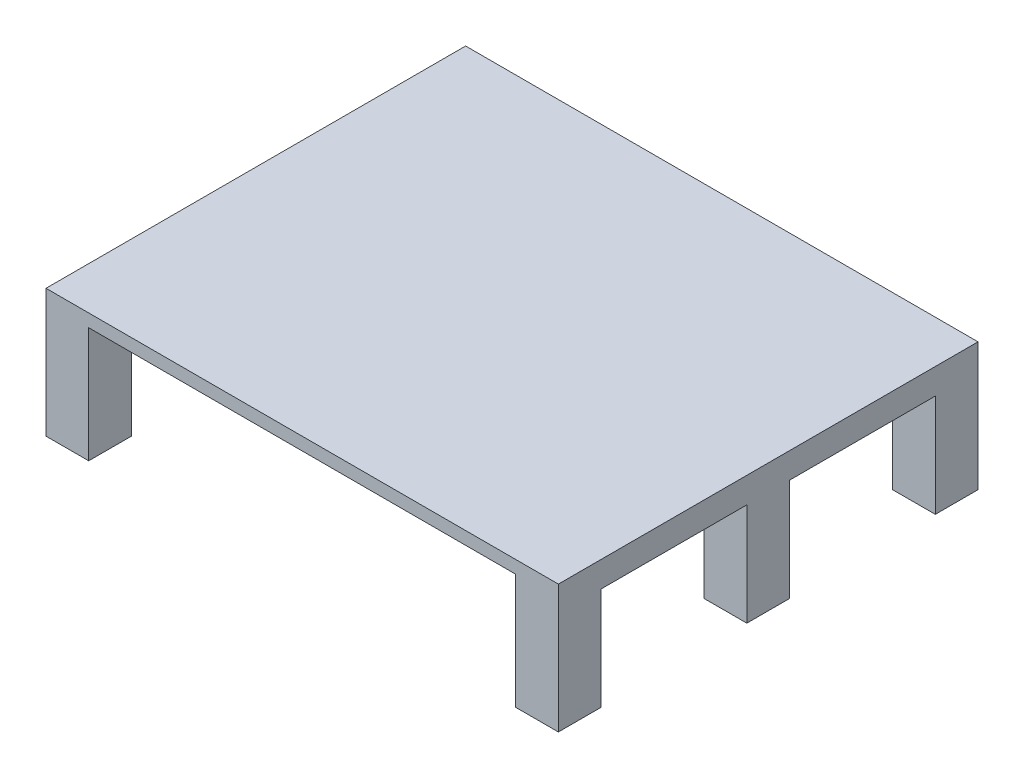
SolidWorks part; units mm, degrees
ref_plane "Front Plane" through (0, 0, 0) normal (0, 0, 1) x (1, 0, 0)
ref_plane "Top Plane" through (0, 0, 0) normal (0, 1, 0) x (1, 0, 0)
ref_plane "Right Plane" through (0, 0, 0) normal (1, 0, 0) x (0, 0, -1)
sketch "Sketch2" plane through (0, 0, 0) normal (0, 0, 1) x (1, 0, 0)
  line L1 (3000, -1500) -> (2500, -1500)
  line L2 (3000, -1500) -> (3000, 0)
  line L3 (3000, 0) -> (-3000, 0)
  line L4 (-3000, -1500) -> (-3000, 0)
  line L5 (0, 0) -> (0, -3054.8137) construction
  line L8 (-2500, -1500) -> (-2500, -150)
  line L9 (-2500, -150) -> (2500, -150)
  line L10 (2500, -1500) -> (2500, -150)
  line L11 (-2500, -1500) -> (-3000, -1500)
  point P0 (0, 0)
  point P6 (0, 0)
  point P11 (2750, -1500)
  dimension "D1" = 1500
  dimension "D2" = 6000
  dimension "D3" = 1350
  dimension "D4" = 5000
extrude "Boss-Extrude1" add sketch "Sketch2" along normal blind 435 and the other way blind 4479
sketch "Sketch3" plane through (3000, 0, 0) normal (1, 0, 0) x (0, 0, -1)
  line L0 (4479, -1500) -> (-435, -1500) construction
  line L1 (65, -1500) -> (1772, -1500)
  line L2 (65, -1500) -> (65, -300)
  line L3 (65, -300) -> (1772, -300)
  line L4 (1772, -1500) -> (1772, -300)
  line L5 (2022, -1500) -> (2022, 353.026) construction
  line L10 (2272, -1500) -> (2272, -300)
  line L11 (3979, -300) -> (2272, -300)
  line L12 (3979, -1500) -> (3979, -300)
  line L13 (3979, -1500) -> (2272, -1500)
  line L14 (-435, -1500) -> (-435, 0) construction
  line L15 (4479, 0) -> (-435, 0) construction
  dimension "D1" = 500
  dimension "D2" = 500
  dimension "D3" = 300
extrude "Cut-Extrude1" cut sketch "Sketch3" against normal through all
